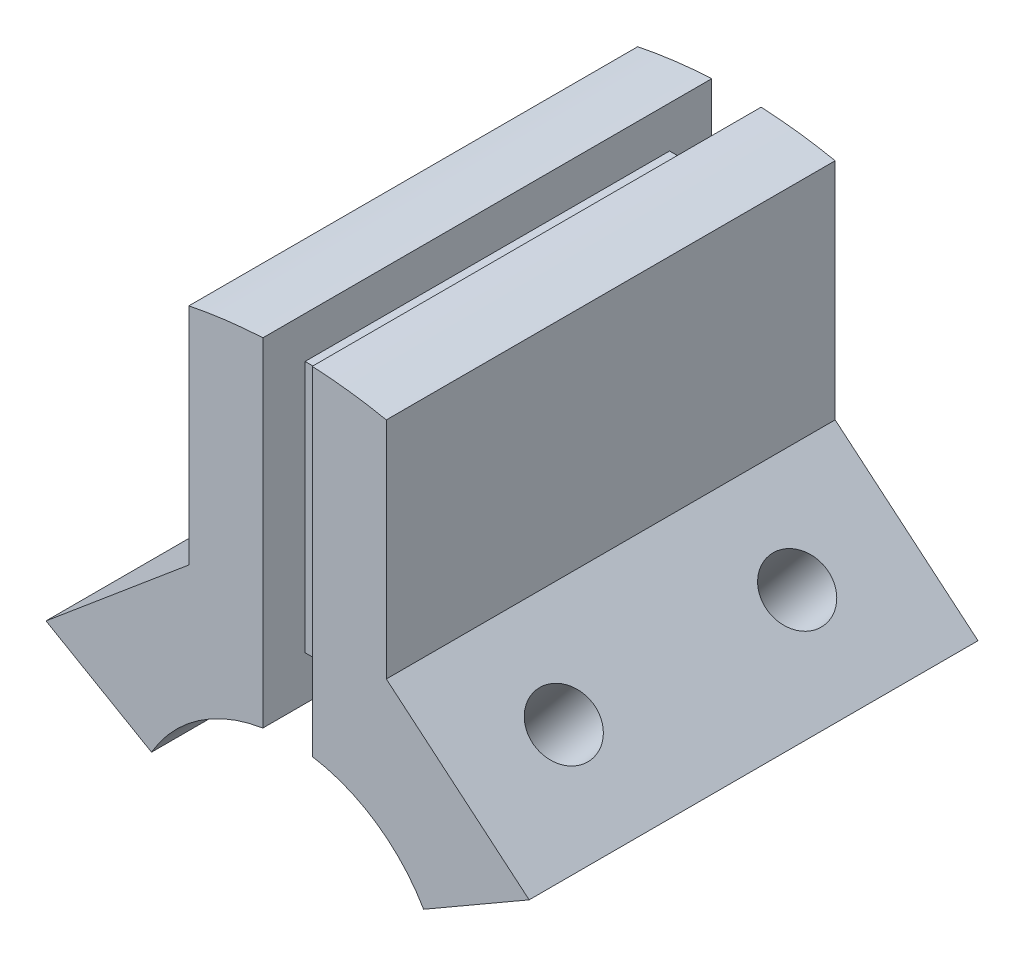
from build123d import *

# Parameters (mm, degrees)
BOSS_EXTRUDE1_DEPTH                   = 25
BOSS_EXTRUDE1_2_DEPTH                 = 25
SKETCH2_W                             = 5.5
SKETCH2_H                             = 28.1
BOSS_EXTRUDE2_DEPTH                   = 20.3
F_6_0MM_BLIND_DOWEL_HOLE1_D           = 6
F_6_0MM_BLIND_DOWEL_HOLE1_ON_FACE_2_D = 6
F_6_0MM_BLIND_DOWEL_HOLE2_D           = 7
F_6_0MM_BLIND_DOWEL_HOLE2_ON_FACE_2_D = 7


with BuildPart() as part:
    # Sketch1 → Boss-Extrude1 (new, symmetric)
    with BuildSketch(Plane.XY):
        with BuildLine():
            Line((-2.75, 54.931206977), (-2.75, 17.282577933))
            ThreePointArc((-2.75, 17.282577933), (-9.917280768, 14.418652578), (-15.155444566, 8.75))
            Line((-15.155444566, 8.75), (-26.911555625, 15.537393885))
            Line((-26.911555625, 15.537393885), (-11, 28.888774341))
            Line((-11, 28.888774341), (-11, 53.888774341))
            ThreePointArc((-11, 53.888774341), (-6.894729251, 54.566131515), (-2.75, 54.931206977))
        make_face()
    extrude(amount=BOSS_EXTRUDE1_DEPTH, both=True)



with BuildPart() as body_2:
    # Sketch1 → Boss-Extrude1 2 (new, symmetric)
    with BuildSketch(Plane.XY):
        with BuildLine():
            Line((11, 28.888774341), (26.911555625, 15.537393885))
            Line((26.911555625, 15.537393885), (15.155444566, 8.75))
            ThreePointArc((15.155444566, 8.75), (9.917280768, 14.418652578), (2.75, 17.282577933))
            Line((2.75, 17.282577933), (2.75, 54.931206977))
            ThreePointArc((2.75, 54.931206977), (6.894729251, 54.566131515), (11, 53.888774341))
            Line((11, 53.888774341), (11, 28.888774341))
        make_face()
    extrude(amount=BOSS_EXTRUDE1_2_DEPTH, both=True)


with BuildPart() as part_1:
    add(part.part)

    add(body_2.part)  # Boss-Extrude2 merges body 2
    # Sketch2 → Boss-Extrude2 (add, symmetric)
    with BuildSketch(Plane.XY):
        with Locations((0, 36.25)):
            Rectangle(SKETCH2_W, SKETCH2_H)
    extrude(amount=BOSS_EXTRUDE2_DEPTH, both=True)

    # Ø6.0mm Blind Dowel Hole1 (through all)
    with Locations(Plane(origin=(-18.769879496, 22.369071322, 13), x_dir=(0.766044443119, 0.642787609687, 0), z_dir=(-0.642787609687, 0.766044443119, 0))):
        with Locations((0, 0)):
            Hole(F_6_0MM_BLIND_DOWEL_HOLE1_D / 2)

    # Ø6.0mm Blind Dowel Hole1 on face 2 (through all)
    with Locations(Plane(origin=(-18.769879496, 22.369071322, -13), x_dir=(0.766044067841, 0.642788056925, 0), z_dir=(-0.642788056925, 0.766044067841, 0))):
        with Locations((0, 0)):
            Hole(F_6_0MM_BLIND_DOWEL_HOLE1_ON_FACE_2_D / 2)

    # Ø6.0mm Blind Dowel Hole2 (through all)
    with Locations(Plane(origin=(18.769879496, 22.369071322, 13), x_dir=(0.766044443119, -0.642787609687, 0), z_dir=(0.642787609687, 0.766044443119, 0))):
        with Locations((0, 0)):
            Hole(F_6_0MM_BLIND_DOWEL_HOLE2_D / 2)

    # Ø6.0mm Blind Dowel Hole2 on face 2 (through all)
    with Locations(Plane(origin=(18.769879496, 22.369071322, -13), x_dir=(0.766044067841, -0.642788056925, 0), z_dir=(0.642788056925, 0.766044067841, 0))):
        with Locations((0, 0)):
            Hole(F_6_0MM_BLIND_DOWEL_HOLE2_ON_FACE_2_D / 2)


solid = part_1.part
